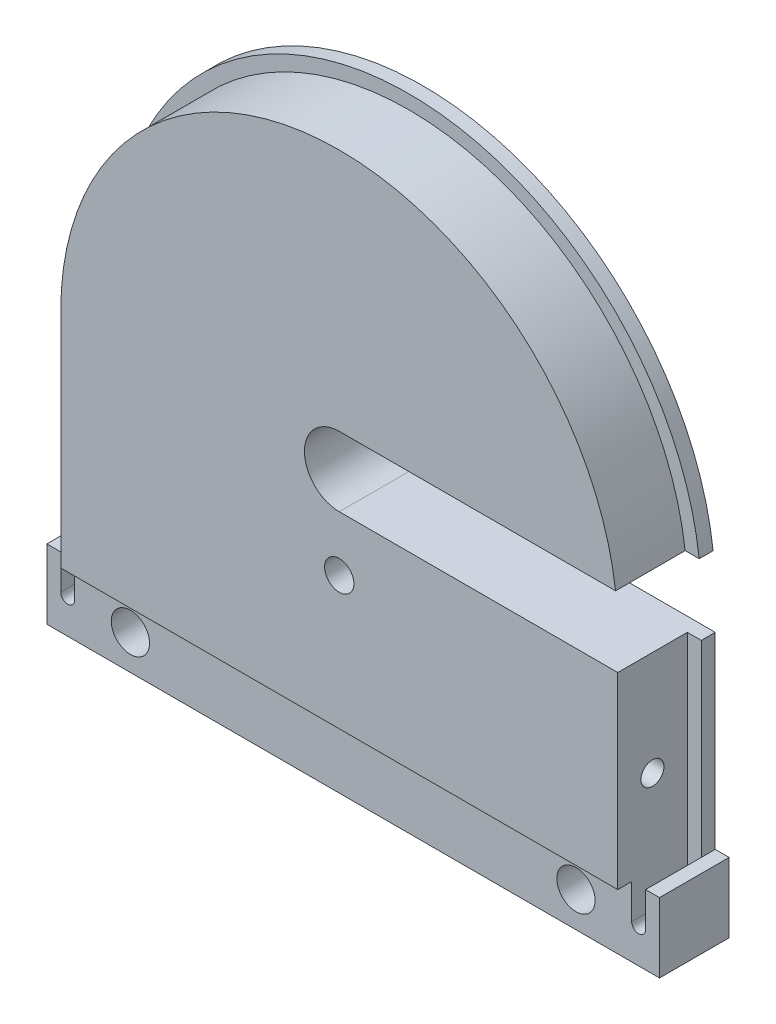
SolidWorks part; units mm, degrees
material "6061 合金"
ref_plane "前视基准面" through (0, 0, 0) normal (0, 0, 1) x (1, 0, 0)
ref_plane "上视基准面" through (0, 0, 0) normal (0, 1, 0) x (1, 0, 0)
ref_plane "右视基准面" through (0, 0, 0) normal (1, 0, 0) x (0, 0, -1)
sketch "草图1" plane through (0, 0, 0) normal (0, 0, 1) x (1, 0, 0)
  line L0 (0, 46.8606) -> (0, -41.5932) construction
  line L1 (-42, 21) -> (42, 21) construction
  line L2 (-44, -11) -> (-44, -21)
  line L3 (-44, -21) -> (44, -21)
  line L4 (44, -11) -> (44, -21)
  line L5 (-42, -11) -> (-44, -11)
  line L7 (-42, 21) -> (-42, -11)
  line L8 (44, -11) -> (42, -11)
  line L13 (42, 21) -> (42, -11)
  arc A0 (42, 21) -> (-42, 21) centre (0, 21) ccw
  point P0 (0, 0)
  point P2 (-44, 21)
  point P4 (44, 21)
  point P10 (-34, 21)
  point P12 (-34, -11)
  point P13 (34, -11)
  point P14 (34, 21)
  dimension "D3" = 84
extrude "凸台-拉伸1" add sketch "草图1" along normal blind 12
sketch "草图2" plane through (0, 0, 12) normal (0, 0, 1) x (1, 0, 0)
  line L5 (-40, 21) -> (-40, -11)
  line L6 (-40, 21) -> (-40, -11)
  line L7 (-40, -11) -> (-42, -11)
  line L8 (40, -11) -> (40, 21)
  line L9 (40, -11) -> (40, 21)
  line L10 (40, -11) -> (42, -11)
  line L11 (42, 21) -> (42, -11)
  line L12 (-42, 21) -> (-42, -11)
  arc A1 (42, 21) -> (-42, 21) centre (0, 21) ccw
  arc A2 (40, 21) -> (-40, 21) centre (0, 21) ccw
  arc A3 (40, 21) -> (-40, 21) centre (0, 21) ccw
  dimension "D1" = 2
  dimension "D2" = 2
  dimension "D3" = 2
extrude "切除-拉伸1" cut sketch "草图2" against normal blind 10
sketch "草图3" plane through (44, 0, 0) normal (1, 0, 0) x (0, 0, -1)
  line L1 (-10, -11) -> (-12, -11)
  line L2 (-10, -21) -> (-10, -11)
  line L3 (-10, -21) -> (-10, -11)
  line L4 (-12, -11) -> (-12, -21)
  line L5 (-12, -21) -> (-10, -21)
  dimension "D1" = 2
extrude "切除-拉伸2" cut sketch "草图3" against normal through all
sketch "草图4" plane through (0, 0, 10) normal (0, 0, 1) x (1, 0, 0)
  line L2 (0, 15.5505) -> (0, -26.6325) construction
  line L3 (-40, -11) -> (-42, -11)
  line L4 (42, -11) -> (42, -16)
  line L5 (-42, -11) -> (-42, -16)
  line L6 (-40, -11) -> (-40, -16)
  line L7 (40, -11) -> (44, -11) construction
  line L8 (40, -11) -> (40, -16)
  line L9 (40, -11) -> (42, -11)
  arc A0 (40, -16) -> (42, -16) centre (41, -16) ccw
  arc A1 (-40, -16) -> (-42, -16) centre (-41, -16) cw
  dimension "D1" = 2
extrude "切除-拉伸3" cut sketch "草图4" against normal blind 8
sketch "草图5" plane through (0, 0, 0) normal (0, 0, -1) x (-1, 0, 0)
  line L0 (-63.4452, 21) -> (61.7305, 21) construction
  line L1 (0, -35.7088) -> (0, 54.4374) construction
  line L2 (0, 26) -> (-46.2639, 26)
  line L3 (-46.2639, 26) -> (-46.2639, 16)
  line L4 (-46.2639, 16) -> (0, 16)
  arc A0 (0, 16) -> (0, 26) centre (0, 21) ccw
  dimension "D1" = 10
extrude "切除-拉伸4" cut sketch "草图5" against normal through all
sketch "草图6" plane through (0, 0, 0) normal (0, 0, -1) x (-1, 0, 0)
  line L1 (0, 13.738) -> (0, -41.0653) construction
  line L2 (44, -16) -> (-44, -16)
  line L3 (44, -16) -> (-44, -16) construction
  line L4 (-32, 13.738) -> (-32, -41.0653) construction
  circle A0 centre (-32, -16) radius 2.75
  circle A1 centre (32, -16) radius 2.75
  dimension "D3" = 5.5
  dimension "D1" = 5
  dimension "D2" = 32
extrude "切除-拉伸5" cut sketch "草图6" against normal through all
sketch "草图7" plane through (0, 0, 0) normal (0, 0, -1) x (-1, 0, 0)
  circle A0 centre (-32, -16) radius 4.5
  circle A1 centre (32, -16) radius 4.5
  dimension "D1" = 9
  dimension "D2" = 9
extrude "切除-拉伸6" cut sketch "草图7" against normal blind 6
sketch "草图8" plane through (-40, 0, 0) normal (-1, 0, 0) x (0, 0, 1)
  line L3 (-5.1424, 1) -> (10, 1) construction
  line L6 (7, -11) -> (7, 21)
  line L7 (7, -11) -> (7, 21) construction
  dimension "D1" = 5
hole_wizard "M4 螺纹孔1" positions "3D草图1" profile "草图9" tap size "M4" standard "GB"
sketch3d "3D草图1"
  line L0 (-40, 1, -5.1424) -> (-40, 1, 10) construction
  line L1 (-40, -11, 7) -> (-40, 21, 7) construction
  point P0 (-40, 1, 7)
sketch "草图9" plane through (-40, 1, 7) normal (0, 1, 0) x (0, 0, 1)
  line L0 (0, 0) -> (0, 10.9914)
  line L1 (0, 10.9914) -> (1.65, 10)
  line L2 (1.65, 10) -> (1.65, 0)
  line L5 (1.65, 0) -> (0, 0)
  line L10 (0, 10.9914) -> (-1.65, 10) construction
  line L11 (0, -6.35) -> (0, 107.95) construction
  dimension "螺纹孔钻头直径" = 3.3
  dimension "螺纹孔钻头深度" = 10
  dimension "导头角度" = 118
cosmetic thread "孔螺蚊线1" parameters "D1"=8, "D2"=4
sketch "草图10" plane through (40, 0, 0) normal (1, 0, 0) x (0, 0, -1)
  line L0 (-17.7717, 1) -> (6.9344, 1) construction
  line L1 (-7, 8.6648) -> (-7, -8.7462) construction
hole_wizard "M4 螺纹孔2" positions "3D草图3" profile "草图12" tap size "M4" standard "GB"
sketch3d "3D草图3"
  line L0 (40, 1, 17.7717) -> (40, 1, -6.9344) construction
  point P0 (40, 1, 7.0154)
sketch "草图12" plane through (40, 1, 7.0154) normal (0, 1, 0) x (0, 0, -1)
  line L0 (0, 0) -> (0, 10.9914)
  line L1 (0, 10.9914) -> (1.65, 10)
  line L2 (1.65, 10) -> (1.65, 0)
  line L5 (1.65, 0) -> (0, 0)
  line L10 (0, 10.9914) -> (-1.65, 10) construction
  line L11 (0, -6.35) -> (0, 107.95) construction
  dimension "螺纹孔钻头直径" = 3.3
  dimension "螺纹孔钻头深度" = 10
  dimension "导头角度" = 118
cosmetic thread "孔螺蚊线2" parameters "D1"=8, "D2"=4
sketch "草图13" plane through (0, 0, 0) normal (0, 0, -1) x (-1, 0, 0)
  line L28 (0, 24.153) -> (0, -36.9918) construction
  line L29 (44, 8) -> (-44, 8)
  line L30 (44, 8) -> (-44, 8) construction
  dimension "D1" = 29
hole_wizard "M5 螺纹孔1" positions "3D草图7" profile "草图17" tap size "M5" standard "GB" end condition through all
sketch3d "3D草图7"
  line L0 (0, 24.153, 0) -> (0, -36.9918, 0) construction
  point P0 (0, 8.0819, 0)
sketch "草图17" plane through (0, 8.0819, 0) normal (1, 0, 0) x (0, 1, 0)
  line L0 (0, 0) -> (0, 12)
  line L1 (0, 12) -> (2.1, 12)
  line L2 (2.1, 12) -> (2.1, 0)
  line L5 (2.1, 0) -> (0, 0)
  line L11 (0, -6.35) -> (0, 107.95) construction
  dimension "通孔螺纹孔钻头直径" = 4.2
  dimension "通孔螺纹孔钻头深度" = 12
cosmetic thread "孔螺蚊线3" parameters "D2"=5
